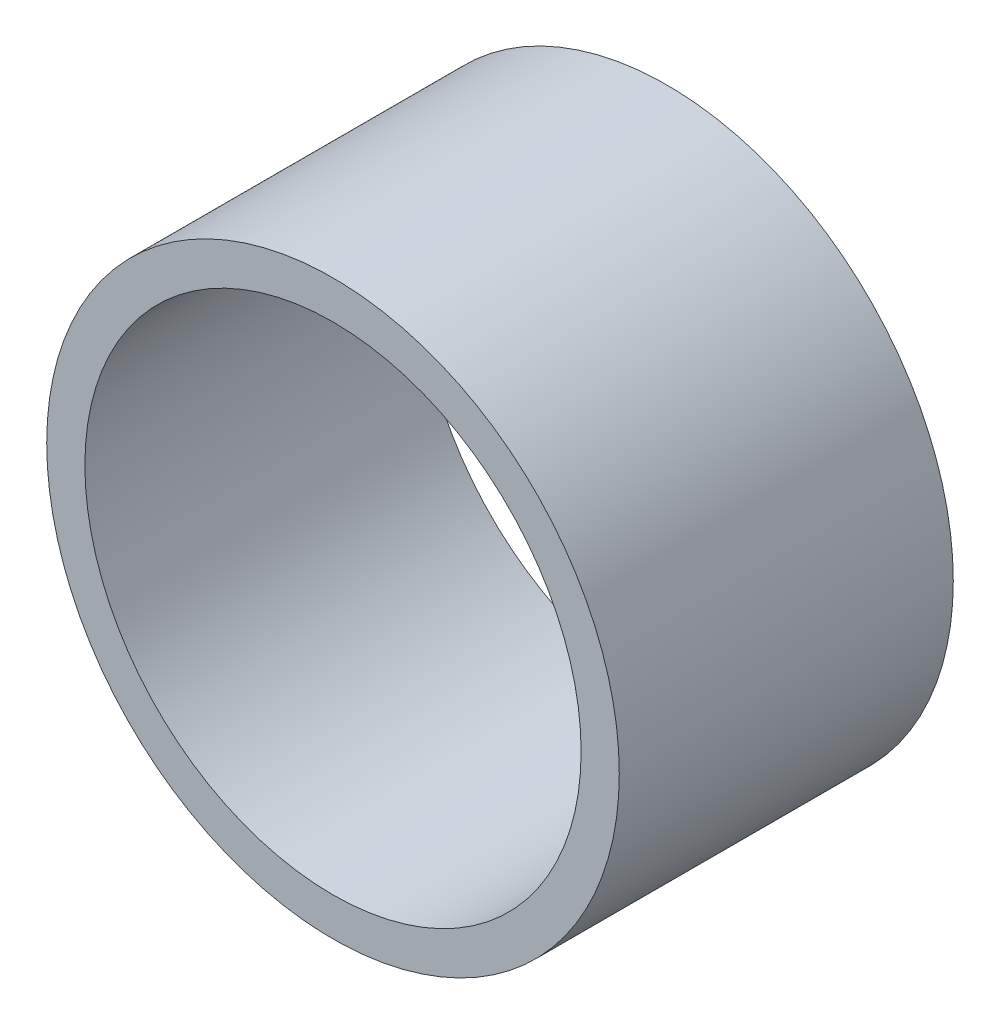
SolidWorks part; units mm, degrees
material "AISI 1045 钢，冷拔"
ref_plane "Front Plane" through (0, 0, 0) normal (0, 0, 1) x (1, 0, 0)
ref_plane "Top Plane" through (0, 0, 0) normal (0, 1, 0) x (1, 0, 0)
ref_plane "Right Plane" through (0, 0, 0) normal (1, 0, 0) x (0, 0, -1)
sketch "Sketch1" plane through (0, 0, 0) normal (0, 0, 1) x (1, 0, 0)
  circle A0 centre (0, 0) radius 13
  circle A1 centre (0, 0) radius 15
  dimension "D1" = 26
  dimension "D2" = 30
extrude "Boss-Extrude1" add sketch "Sketch1" along normal blind 17.5
